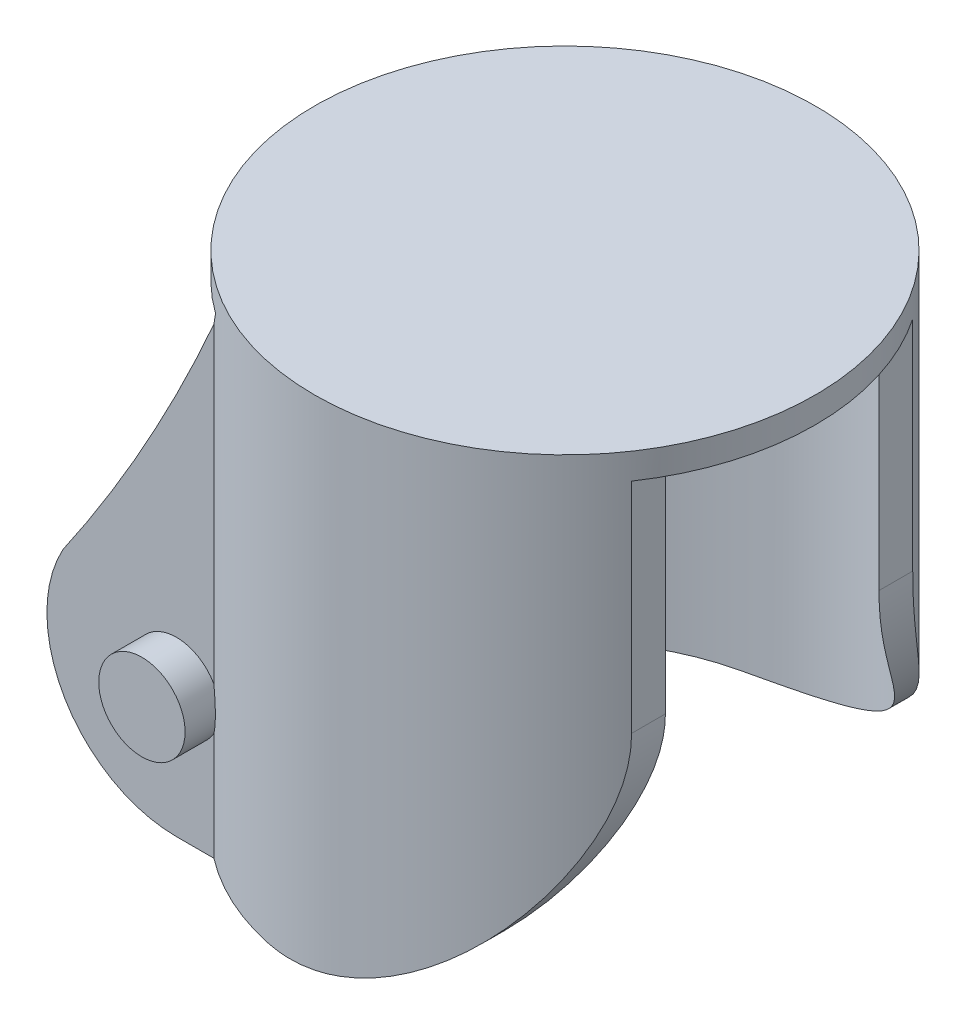
from build123d import *

# Parameters (mm, degrees)
EXTRUDE_1_DEPTH          = 100
SKETCH_3_W               = 42
SKETCH_3_H               = 100
CUT_EXTRUDE_1_DEPTH      = 100
CUT_EXTRUDE_START        = -100
SKETCH_4_R               = 27
CUT_EXTRUDE_2_DEPTH      = 100
CUT_EXTRUDE_3_DEPTH      = 100
CUT_EXTRUDE_3_DEPTH_BACK = 100
SKETCH_6_R               = 5
EXTRUDE_2_DEPTH          = 4
CUT_EXTRUDE_START_2      = -10
SKETCH_8_R               = 6
CUT_EXTRUDE_4_DEPTH      = 10


with BuildPart() as part:
    # 草图1 → 旋转1 (revolve)
    with BuildSketch(Plane(origin=(0, 0, 0), x_dir=(0, 0, -1), z_dir=(1, 0, 0))):
        Polygon((0, -18.2), (-27, -18.2), (-27, -116.2), (-29, -116.2), (-29, -16.2), (0, -16.2), align=None)
    revolve(axis=Axis((0, -16.2, 0), (0, -1, 0)))

    # 草图2 → 凸台-拉伸1 (add)
    with BuildSketch(Plane(origin=(0, 0, 0), x_dir=(0, 0, -1), z_dir=(1, 0, 0))):
        Polygon((-23, -19.2), (-23, -119.2), (-21, -119.2), (-21, -21.2), (21, -21.2), (21, -119.2), (23, -119.2), (23, -19.2), align=None)
    extrude(amount=-EXTRUDE_1_DEPTH)

    # 草图3 → 切除-拉伸1 (cut)
    with BuildSketch(Plane(origin=(0, 0, 0), x_dir=(0, 0, -1), z_dir=(1, 0, 0))):
        with Locations((0, -69.2)):
            Rectangle(SKETCH_3_W, SKETCH_3_H)
    extrude(amount=-CUT_EXTRUDE_1_DEPTH, mode=Mode.SUBTRACT)

    # 草图4 → 切除-拉伸2 (cut)
    with BuildSketch(Plane(origin=(0, -18.2, 0), x_dir=(1, 0, 0), z_dir=(0, 1, 0)).offset(CUT_EXTRUDE_START)):
        with Locations(Location((0, 0, 0), (0, 0, 270))):
            Circle(SKETCH_4_R)
    extrude(amount=CUT_EXTRUDE_2_DEPTH, mode=Mode.SUBTRACT)

    # 草图5 → 切除-拉伸3 (cut, two sides: drawn at the far end of the back side and taken through both)
    with BuildSketch(Plane.XY.offset(-CUT_EXTRUDE_3_DEPTH_BACK)):
        with BuildLine():
            Line((-120, -19.2), (-120, -120))
            Line((-120, -120), (29, -120))
            Line((29, -120), (29, -19.2))
            Line((29, -19.2), (24, -19.2))
            Line((24, -19.2), (24, -44.5))
            ThreePointArc((24, -44.5), (15.213203436, -65.713203436), (-6, -74.5))
            Line((-6, -74.5), (-22, -74.5))
            ThreePointArc((-22, -74.5), (-34.915252207, -67.128647352), (-35.136787274, -52.25950139))
            ThreePointArc((-35.136787274, -52.25950139), (-25.194624928, -36.188092129), (-16.915644702, -19.2))
            Line((-16.915644702, -19.2), (-120, -19.2))
        make_face()
    extrude(amount=CUT_EXTRUDE_3_DEPTH + CUT_EXTRUDE_3_DEPTH_BACK, mode=Mode.SUBTRACT)

    # 草图6 → 凸台-拉伸2 (add)
    with BuildSketch(Plane.XY.offset(23)):
        with Locations(Location((-22, -59.5, 0), (0, 0, 29.854118281))):
            Circle(SKETCH_6_R)
    extrude(amount=EXTRUDE_2_DEPTH)

    # 草图7 → 旋转2 (revolve)
    with BuildSketch(Plane(origin=(-22, 0, 0), x_dir=(0, 0, -1), z_dir=(1, 0, 0)), mode=Mode.PRIVATE) as revolve_2_sk:
        with BuildLine():
            Line((23, -59.5), (23, -53.5))
            Line((23, -53.5), (28, -53.5))
            ThreePointArc((28, -53.5), (28.688549603, -54.580756174), (29, -55.823790008))
            Line((29, -55.823790008), (29, -59.5))
            Line((29, -59.5), (23, -59.5))
        make_face()
    revolve(revolve_2_sk.sketch.rotate(Axis((-22, -59.5, -29), (0, 0, 1)), 90), axis=Axis((-22, -59.5, -29), (0, 0, 1)))

    # 草图8 → 切除-拉伸4 (cut)
    with BuildSketch(Plane.XY.offset(-23).offset(CUT_EXTRUDE_START_2)):
        with Locations((-22, -59.5)):
            Circle(SKETCH_8_R)
        Polygon((-27, -56.613248654), (-27, -62.386751346), (-22, -65.273502692), (-17, -62.386751346), (-17, -56.613248654), (-22, -53.726497308), align=None, mode=Mode.SUBTRACT)
    extrude(amount=CUT_EXTRUDE_4_DEPTH, mode=Mode.SUBTRACT)


solid = part.part
